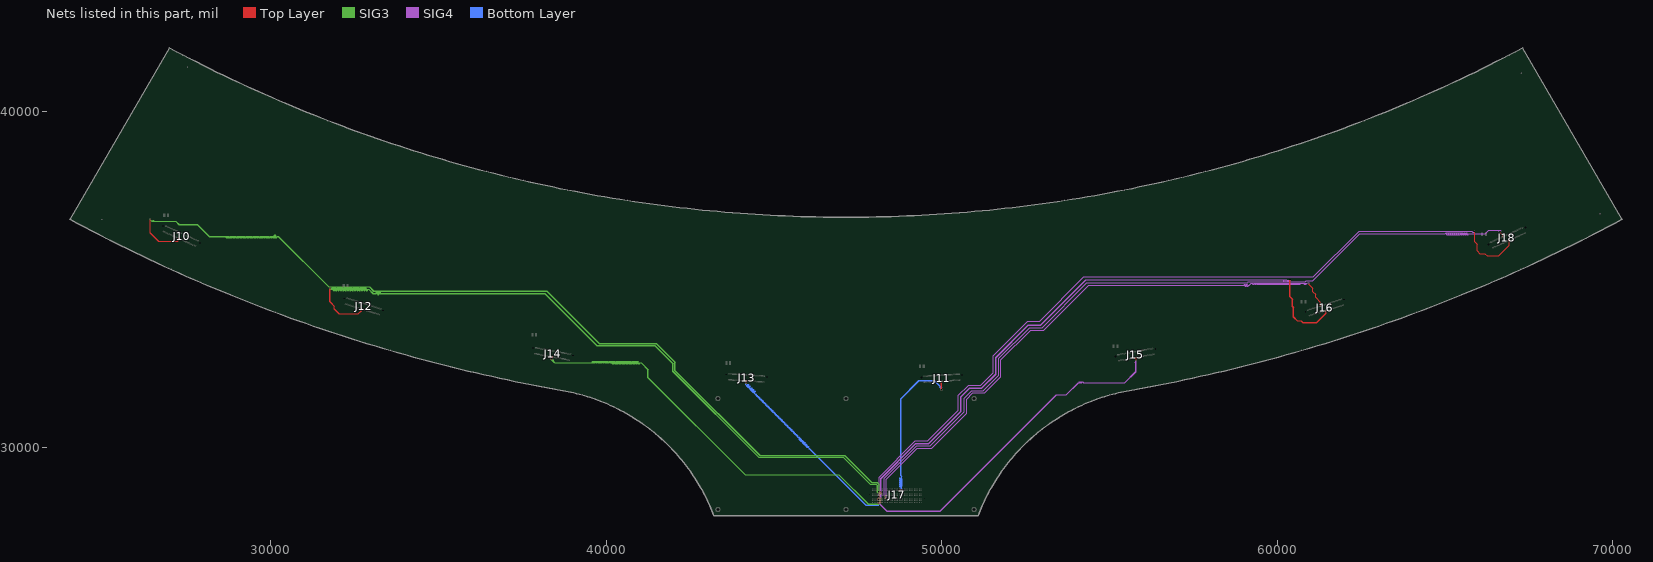
[diagram p0: the nets of this part, all layers, seen from the top]
# Altium PCB MISC86329.PcbDoc (part 9 of 11)
Units mil, origin at the board's own origin, x right, y up, seen from the top; angles counter-clockwise.
Board outline 46247.15 x 13937.21 mil, 6 copper layers (Top Layer, GND2, SIG3, SIG4, POWER5, Bottom Layer); 17 components, 210 nets, 908 pads, 1109 vias.

## Via types
v1: diameter 24, hole 12, Top Layer to Bottom Layer, 684 vias
v2: diameter 18, hole 9, Top Layer to Bottom Layer, 425 vias

## Nets (pads, with @x,y where several pads share a name; then routed paths per layer and width w, separated by ;. In a path a pad name is that pad's centre, name@x,y a point inside that pad or via, vN(x,y) a via of type N, cw(c..) or ccw(c..) an arc to the next point about the centre after c; other vN are vias at no path point) (continued)
DATAIN6P_CH6: J16.28 J17.D22 | length 18290.3
  Top Layer w5: v2(48314.09,28495) J17.D22@48337.89,28518.8 ; 60949,34880.5 60949,34846 61055,34740 61055,34648 61141,34562 61141,34474 61286,34329 61286,34220.6 J16.28@61285.27,34219.87
  SIG4 w5: v2(48314.09,28495) 48344,28524.91 48344,29053 49268,29977 49697.14,29977 50747,31026.86 50747,31446 50928,31627 51285.14,31627 51764,32105.86 51764,32612 52653,33501 53046.14,33501 54377.14,34832 59009.14,34832 59019.57,34842.43 59019.57,34857.43 59024.14,34862 59035,34862 59039.57,34857.43 59039.57,34812.43 59050,34802 59069.14,34802 59079.57,34812.43 59079.57,34857.43 59084.14,34862 59095,34862 59099.57,34857.43 59099.57,34812.43 59110,34802 59129.14,34802 59139.57,34812.43 59139.57,34827.43 59144.14,34832 59159.14,34832 59218.14,34891 59260.93,34891 59265.5,34886.43 59265.5,34871.43 59275.93,34861 59295.07,34861 59305.5,34871.43 59305.5,34886.43 59310.07,34891 59320.93,34891 59325.5,34886.43 59325.5,34871.43 59335.93,34861 59355.07,34861 59365.5,34871.43 59365.5,34886.43 59370.07,34891 59380.93,34891 59385.5,34886.43 59385.5,34871.43 59395.93,34861 59415.07,34861 59425.5,34871.43 59425.5,34886.43 59430.07,34891 59440.93,34891 59445.5,34886.43 59445.5,34871.43 59455.93,34861 59475.07,34861 59485.5,34871.43 59485.5,34886.43 59490.07,34891 59500.93,34891 59505.5,34886.43 59505.5,34871.43 59515.93,34861 59535.07,34861 59545.5,34871.43 59545.5,34886.43 59550.07,34891 59560.93,34891 59565.5,34886.43 59565.5,34871.43 59575.93,34861 59595.07,34861 59605.5,34871.43 59605.5,34886.43 59610.07,34891 59620.93,34891 59625.5,34886.43 59625.5,34871.43 59635.93,34861 59655.07,34861 59665.5,34871.43 59665.5,34886.43 59670.07,34891 59680.93,34891 59685.5,34886.43 59685.5,34871.43 59695.93,34861 59715.07,34861 59725.5,34871.43 59725.5,34886.43 59730.07,34891 59740.93,34891 59745.5,34886.43 59745.5,34871.43 59755.93,34861 59775.07,34861 59785.5,34871.43 59785.5,34886.43 59790.07,34891 59800.93,34891 59805.5,34886.43 59805.5,34871.43 59815.93,34861 59835.07,34861 59845.5,34871.43 59845.5,34886.43 59850.07,34891 59860.93,34891 59865.5,34886.43 59865.5,34871.43 59875.93,34861 59895.07,34861 59905.5,34871.43 59905.5,34886.43 59910.07,34891 59920.93,34891 59925.5,34886.43 59925.5,34871.43 59935.93,34861 59955.07,34861 59965.5,34871.43 59965.5,34886.43 59970.07,34891 59980.93,34891 59985.5,34886.43 59985.5,34871.43 59995.93,34861 60015.07,34861 60025.5,34871.43 60025.5,34886.43 60030.07,34891 60040.93,34891 60045.5,34886.43 60045.5,34871.43 60055.93,34861 60075.07,34861 60085.5,34871.43 60085.5,34886.43 60090.07,34891 60100.93,34891 60105.5,34886.43 60105.5,34871.43 60115.93,34861 60135.07,34861 60145.5,34871.43 60145.5,34886.43 60150.07,34891 60160.93,34891 60165.5,34886.43 60165.5,34871.43 60175.93,34861 60195.07,34861 60205.5,34871.43 60205.5,34886.43 60210.07,34891 60220.93,34891 60225.5,34886.43 60225.5,34871.43 60235.93,34861 60255.07,34861 60265.5,34871.43 60265.5,34886.43 60270.07,34891 60280.93,34891 60285.5,34886.43 60285.5,34871.43 60295.93,34861 60315.07,34861 60325.5,34871.43 60325.5,34886.43 60330.07,34891 60340.93,34891 60345.5,34886.43 60345.5,34871.43 60355.93,34861 60375.07,34861 60385.5,34871.43 60385.5,34886.43 60390.07,34891 60400.93,34891 60405.5,34886.43 60405.5,34871.43 60415.93,34861 60435.07,34861 60445.5,34871.43 60445.5,34886.43 60450.07,34891 60460.93,34891 60465.5,34886.43 60465.5,34871.43 60475.93,34861 60495.07,34861 60505.5,34871.43 60505.5,34886.43 60510.07,34891 60520.93,34891 60525.5,34886.43 60525.5,34871.43 60535.93,34861 60555.07,34861 60565.5,34871.43 60565.5,34886.43 60570.07,34891 60580.93,34891 60585.5,34886.43 60585.5,34871.43 60595.93,34861 60615.07,34861 60625.5,34871.43 60625.5,34886.43 60630.07,34891 60640.93,34891 60645.5,34886.43 60645.5,34871.43 60655.93,34861 60675.07,34861 60685.5,34871.43 60685.5,34886.43 60690.07,34891 60703,34891 60791,34891 60796,34886 60796,34873.23 60801,34868.23 60811,34868.23 60816,34873.23 60816,34886 60821,34891 60831,34891 60836,34886 60836,34873.23 60841,34868.23 60851,34868.23 60856,34873.23 60856,34886 60861,34891 60866,34891 60882.14,34891 60908.14,34917 60941,34917 60949,34909 60949,34893 v2@60943,34887
  other v2: 60942.5,34887
DATAIN6P_CH7: J17.E22 J18.28 | length 23893.1
  Top Layer w5: v2(48314.09,28545) J17.E22@48337.89,28568.8 ; 66665,36423.5 66665,36390 66717.39,36337.61 J18.28@66717.39,36281.33
  SIG4 w5: v2(48314.09,28545) 48294.09,28565 48294.09,29081.09 49260,30047 49655.14,30047 50669,31060.86 50669,31464.86 50895.14,31691 51236.14,31691 51698,32152.86 51698,32656 52618,33576 52990.14,33576 54328.14,34914 59117.14,34914 59137.14,34934 60830.14,34934 60868.14,34972 61057.14,34972 62452.14,36367 65008,36367 65038,36397 65049.43,36397 65054,36392.43 65054,36347.43 65064.43,36337 65083.57,36337 65094,36347.43 65094,36392.43 65098.57,36397 65109.43,36397 65114,36392.43 65114,36347.43 65124.43,36337 65143.57,36337 65154,36347.43 65154,36392.43 65158.57,36397 65169.43,36397 65174,36392.43 65174,36347.43 65184.43,36337 65203.57,36337 65214,36347.43 65214,36392.43 65218.57,36397 65229.43,36397 65234,36392.43 65234,36347.43 65244.43,36337 65263.57,36337 65274,36347.43 65274,36392.43 65278.57,36397 65289.43,36397 65294,36392.43 65294,36347.43 65304.43,36337 65323.57,36337 65334,36347.43 65334,36392.43 65338.57,36397 65349.43,36397 65354,36392.43 65354,36347.43 65364.43,36337 65383.57,36337 65394,36347.43 65394,36392.43 65398.57,36397 65409.43,36397 65414,36392.43 65414,36347.43 65424.43,36337 65443.57,36337 65454,36347.43 65454,36392.43 65458.57,36397 65469.43,36397 65474,36392.43 65474,36347.43 65484.43,36337 65503.57,36337 65514,36347.43 65514,36392.43 65518.57,36397 65529.43,36397 65534,36392.43 65534,36347.43 65544.43,36337 65563.57,36337 65574,36347.43 65574,36392.43 65578.57,36397 65589.43,36397 65594,36392.43 65594,36347.43 65604.43,36337 65623.57,36337 65634,36347.43 65634,36392.43 65638.57,36397 65649.43,36397 65654,36392.43 65654,36347.43 65664.43,36337 65683.57,36337 65694,36347.43 65694,36362.43 65698.57,36367 66189.14,36367 66304.14,36482 66581,36482 66586,36477 66586,36461.86 66591,36456.86 66601,36456.86 66606,36461.86 66606,36477 66611,36482 66637,36482 66665,36454 66665,36437 v2@66660,36432
  other v2: 66658.5,36430
DATAIN7N_CH0: J10.35 J17.G26 | length 28227.4
  Top Layer w5: v2(26406.5,36813) 26413,36806.5 26413,36389.86 26659.86,36143 27230.14,36143 27272.65,36185.51 27272.65,36199.68 J10.35@27291.29,36218.32 ; v2(48114.09,28692.61) J17.G26@48137.89,28668.8
  SIG3 w5: 26413,36806.5 26413,36783 26459,36737 27176,36737 27272,36641 27815.86,36641 27868.86,36588 ; 27869,36588 27868.86,36588 ; v2(48114.09,28692.61) 48134.09,28712.61 48134.09,28890.77 48073.86,28951 47916.86,28951 47107.86,29760 44584.86,29760 42053,32291.86 42053,32541 41497,33097 39794.86,33097 38227.86,34664 33067.86,34664 32946.86,34785 31734,34785 30233,36286 30200.32,36286 30194.5,36280.18 30194.5,36257.84 30182.82,36246.16 30161.18,36246.16 30149.5,36257.84 30149.5,36320.02 30143.68,36325.84 30130.32,36325.84 30124.5,36320.02 30124.5,36257.84 30112.82,36246.16 30091.18,36246.16 30079.5,36257.84 30079.5,36280.18 30073.68,36286 30060.32,36286 30054.5,36280.18 30054.5,36257.84 30042.82,36246.16 30021.18,36246.16 30009.5,36257.84 30009.5,36280.18 30003.68,36286 29990.32,36286 29984.5,36280.18 29984.5,36257.84 29972.82,36246.16 29951.18,36246.16 29939.5,36257.84 29939.5,36280.18 29933.68,36286 29920.32,36286 29914.5,36280.18 29914.5,36257.84 29902.82,36246.16 29881.18,36246.16 29869.5,36257.84 29869.5,36280.18 29863.68,36286 29850.32,36286 29844.5,36280.18 29844.5,36257.84 29832.82,36246.16 29811.18,36246.16 29799.5,36257.84 29799.5,36280.18 29793.68,36286 29780.32,36286 29774.5,36280.18 29774.5,36257.84 29762.82,36246.16 29741.18,36246.16 29729.5,36257.84 29729.5,36280.18 29723.68,36286 29710.32,36286 29704.5,36280.18 29704.5,36257.84 29692.82,36246.16 29671.18,36246.16 29659.5,36257.84 29659.5,36280.18 29653.68,36286 29640.32,36286 29634.5,36280.18 29634.5,36257.84 29622.82,36246.16 29601.18,36246.16 29589.5,36257.84 29589.5,36280.18 29583.68,36286 29570.32,36286 29564.5,36280.18 29564.5,36257.84 29552.82,36246.16 29531.18,36246.16 29519.5,36257.84 29519.5,36280.18 29513.68,36286 29500.32,36286 29494.5,36280.18 29494.5,36257.84 29482.82,36246.16 29461.18,36246.16 29449.5,36257.84 29449.5,36280.18 29443.68,36286 29430.32,36286 29424.5,36280.18 29424.5,36257.84 29412.82,36246.16 29391.18,36246.16 29379.5,36257.84 29379.5,36280.18 29373.68,36286 29360.32,36286 29354.5,36280.18 29354.5,36257.84 29342.82,36246.16 29321.18,36246.16 29309.5,36257.84 29309.5,36280.18 29303.68,36286 29290.32,36286 29284.5,36280.18 29284.5,36257.84 29272.82,36246.16 29251.18,36246.16 29239.5,36257.84 29239.5,36280.18 29233.68,36286 29220.32,36286 29214.5,36280.18 29214.5,36257.84 29202.82,36246.16 29181.18,36246.16 29169.5,36257.84 29169.5,36280.18 29163.68,36286 29150.32,36286 29144.5,36280.18 29144.5,36257.84 29132.82,36246.16 29111.18,36246.16 29099.5,36257.84 29099.5,36280.18 29093.68,36286 29080.32,36286 29074.5,36280.18 29074.5,36257.84 29062.82,36246.16 29041.18,36246.16 29029.5,36257.84 29029.5,36280.18 29023.68,36286 29010.32,36286 29004.5,36280.18 29004.5,36257.84 28992.82,36246.16 28971.18,36246.16 28959.5,36257.84 28959.5,36280.18 28953.68,36286 28940.32,36286 28934.5,36280.18 28934.5,36257.84 28922.82,36246.16 28901.18,36246.16 28889.5,36257.84 28889.5,36280.18 28883.68,36286 28870.32,36286 28864.5,36280.18 28864.5,36257.84 28852.82,36246.16 28831.18,36246.16 28819.5,36257.84 28819.5,36280.18 28813.68,36286 28800.32,36286 28794.5,36280.18 28794.5,36257.84 28782.82,36246.16 28761.18,36246.16 28749.5,36257.84 28749.5,36280.18 28743.68,36286 28730.32,36286 28724.5,36280.18 28724.5,36257.84 28712.82,36246.16 28691.18,36246.16 28679.5,36257.84 28679.5,36280.18 28673.68,36286 28170.86,36286 27868.86,36588
DATAIN7N_CH1: J12.35 J17.F26 | length 23092.2
  Top Layer w5: v2(31758.5,34755) 31765,34748.5 31765,34343.86 31895,34213.86 31895,34128.86 32039.86,33984 32619.14,33984 32713.22,34078.08 32713.22,34102.04 J12.35@32733.25,34122.07 ; v2(48114.09,28642.61) J17.F26@48137.89,28618.8
  SIG3 w5: v2(31758.5,34755) 31765,34748.5 31765,34729.86 31780.93,34713.93 ; 31781,34714 31783,34712 31830.82,34712 31842.5,34723.68 31842.5,34746.18 31848.32,34752 31861.68,34752 31867.5,34746.18 31867.5,34683.68 31879.18,34672 31900.82,34672 31912.5,34683.68 31912.5,34746.18 31918.32,34752 31931.68,34752 31937.5,34746.18 31937.5,34683.68 31949.18,34672 31970.82,34672 31982.5,34683.68 31982.5,34746.18 31988.32,34752 32001.68,34752 32007.5,34746.18 32007.5,34683.68 32019.18,34672 32040.82,34672 32052.5,34683.68 32052.5,34746.18 32058.32,34752 32071.68,34752 32077.5,34746.18 32077.5,34683.68 32089.18,34672 32110.82,34672 32122.5,34683.68 32122.5,34746.18 32128.32,34752 32141.68,34752 32147.5,34746.18 32147.5,34683.68 32159.18,34672 32180.82,34672 32192.5,34683.68 32192.5,34746.18 32198.32,34752 32211.68,34752 32217.5,34746.18 32217.5,34683.68 32229.18,34672 32250.82,34672 32262.5,34683.68 32262.5,34746.18 32268.32,34752 32281.68,34752 32287.5,34746.18 32287.5,34683.68 32299.18,34672 32320.82,34672 32332.5,34683.68 32332.5,34746.18 32338.32,34752 32351.68,34752 32357.5,34746.18 32357.5,34683.68 32369.18,34672 32390.82,34672 32402.5,34683.68 32402.5,34746.18 32408.32,34752 32421.68,34752 32427.5,34746.18 32427.5,34683.68 32439.18,34672 32460.82,34672 32472.5,34683.68 32472.5,34746.18 32478.32,34752 32491.68,34752 32497.5,34746.18 32497.5,34683.68 32509.18,34672 32530.82,34672 32542.5,34683.68 32542.5,34746.18 32548.32,34752 32561.68,34752 32567.5,34746.18 32567.5,34683.68 32579.18,34672 32600.82,34672 32612.5,34683.68 32612.5,34746.18 32618.32,34752 32631.68,34752 32637.5,34746.18 32637.5,34683.68 32649.18,34672 32670.82,34672 32682.5,34683.68 32682.5,34746.18 32688.32,34752 32701.68,34752 32707.5,34746.18 32707.5,34683.68 32719.18,34672 32740.82,34672 32752.5,34683.68 32752.5,34746.18 32758.32,34752 32771.68,34752 32777.5,34746.18 32777.5,34683.68 32789.18,34672 32810.82,34672 32822.5,34683.68 32822.5,34746.18 32828.32,34752 32841.68,34752 32847.5,34746.18 32847.5,34683.68 32859.18,34672 32880.82,34672 32892.5,34683.68 32892.5,34706.18 32898.32,34712 32930.86,34712 33052.86,34590 33155.82,34590 33167.5,34601.68 33167.5,34621.05 33173.32,34626.87 33186.68,34626.87 33192.5,34621.05 33192.5,34564.81 33204.18,34553.13 33225.82,34553.13 33237.5,34564.81 33237.5,34621.05 33243.32,34626.87 33256.68,34626.87 33262.5,34621.05 33262.5,34601.68 33274.18,34590 38166.86,34590 39724.86,33032 41451,33032 41987,32496 41987,32265.86 44547.86,29705 47065.86,29705 47870.86,28900 48045.86,28900 48086,28859.86 48086,28670.69 48104.66,28652.04 v2(48114.09,28642.61)
DATAIN7N_CH2: J14.35 J17.B26 | length 13805.7
  Top Layer w5: v2@38383.5,32646 38383.5,32645.67 v2(38383.83,32646) ; v2@38384,32646 38377,32653 38377,32676 38390.12,32689.12 J14.35@38390.12,32704.64 ; v2(48114.09,28395) J17.B26@48137.89,28418.8
  SIG3 w5: v2@38382,32643 38377,32638 38377,32625.14 38390.07,32612.07 38394.49,32607.65 38403.33,32607.65 38409.83,32614.15 38418.67,32614.15 38427.51,32605.31 38427.51,32596.47 38421.01,32589.97 38421.01,32581.14 38455.07,32547.07 38469.14,32533 39580.68,32533 39586.5,32538.82 39586.5,32561.32 39598.18,32573 39619.82,32573 39631.5,32561.32 39631.5,32538.82 39637.32,32533 39650.68,32533 39656.5,32538.82 39656.5,32561.32 39668.18,32573 39689.82,32573 39701.5,32561.32 39701.5,32538.82 39707.32,32533 39720.68,32533 39726.5,32538.82 39726.5,32561.32 39738.18,32573 39759.82,32573 39771.5,32561.32 39771.5,32538.82 39777.32,32533 39790.68,32533 39796.5,32538.82 39796.5,32561.32 39808.18,32573 39829.82,32573 39841.5,32561.32 39841.5,32538.82 39847.32,32533 39860.68,32533 39866.5,32538.82 39866.5,32561.32 39878.18,32573 39899.82,32573 39911.5,32561.32 39911.5,32538.82 39917.32,32533 39930.68,32533 39936.5,32538.82 39936.5,32561.32 39948.18,32573 39969.82,32573 39981.5,32561.32 39981.5,32538.82 39987.32,32533 40000.68,32533 40006.5,32538.82 40006.5,32561.32 40018.18,32573 40039.82,32573 40051.5,32561.32 40051.5,32538.82 40057.32,32533 40070.68,32533 40076.5,32538.82 40076.5,32561.32 40088.18,32573 40109.82,32573 40121.5,32561.32 40121.5,32538.82 40127.32,32533 40140.68,32533 40146.5,32538.82 40146.5,32561.32 40158.18,32573 40179.82,32573 40191.5,32561.32 40191.5,32508.82 40197.32,32503 40210.68,32503 40216.5,32508.82 40216.5,32561.32 40228.18,32573 40249.82,32573 40261.5,32561.32 40261.5,32508.82 40267.32,32503 40280.68,32503 40286.5,32508.82 40286.5,32561.32 40298.18,32573 40319.82,32573 40331.5,32561.32 40331.5,32508.82 40337.32,32503 40350.68,32503 40356.5,32508.82 40356.5,32561.32 40368.18,32573 40389.82,32573 40401.5,32561.32 40401.5,32508.82 40407.32,32503 40420.68,32503 40426.5,32508.82 40426.5,32561.32 40438.18,32573 40459.82,32573 40471.5,32561.32 40471.5,32508.82 40477.32,32503 40490.68,32503 40496.5,32508.82 40496.5,32561.32 40508.18,32573 40529.82,32573 40541.5,32561.32 40541.5,32508.82 40547.32,32503 40560.68,32503 40566.5,32508.82 40566.5,32561.32 40578.18,32573 40599.82,32573 40611.5,32561.32 40611.5,32508.82 40617.32,32503 40630.68,32503 40636.5,32508.82 40636.5,32561.32 40648.18,32573 40669.82,32573 40681.5,32561.32 40681.5,32508.82 40687.32,32503 40700.68,32503 40706.5,32508.82 40706.5,32561.32 40718.18,32573 40739.82,32573 40751.5,32561.32 40751.5,32508.82 40757.32,32503 40770.68,32503 40776.5,32508.82 40776.5,32561.32 40788.18,32573 40809.82,32573 40821.5,32561.32 40821.5,32508.82 40827.32,32503 40840.68,32503 40846.5,32508.82 40846.5,32561.32 40858.18,32573 40879.82,32573 40891.5,32561.32 40891.5,32508.82 40897.32,32503 40910.68,32503 40916.5,32508.82 40916.5,32561.32 40928.18,32573 40949.82,32573 40961.5,32561.32 40961.5,32508.82 40967.32,32503 40980.68,32503 40986.5,32508.82 40986.5,32521.32 40998.18,32533 41048,32533 41255,32326 41255,32084 44144,29195 46934,29195 47809,28320 48118,28320 48134,28336 48134,28375.09 v2(48114.09,28395)
DATAIN7N_CH3: J13.35 J17.A26 | length 7746.6
  Top Layer w5: 44166.84,31931.5 44166.84,31949.28 44177.55,31960 J13.35@44177.55,31987.19 ; v2(48114.09,28345) J17.A26@48137.89,28368.8
  Bottom Layer w5: v2@44172,31923 44167,31918 44167,31870.14 44183.03,31854.11 44188.79,31854.11 44221.32,31886.64 44235.36,31886.64 44253.14,31868.86 44253.14,31854.82 44220.61,31822.29 44220.61,31816.53 44232.53,31804.61 44238.29,31804.61 44270.81,31837.14 44284.85,31837.14 44302.63,31819.36 44302.63,31805.32 44270.11,31772.79 44270.11,31767.04 44282.03,31755.12 44287.78,31755.12 44320.31,31787.64 44334.35,31787.64 44352.13,31769.86 44352.13,31755.82 44319.6,31723.3 44319.6,31717.54 44331.52,31705.62 44337.28,31705.62 44369.81,31738.15 44383.85,31738.15 44401.63,31720.37 44401.63,31706.33 44369.1,31673.8 44369.1,31668.04 44381.02,31656.12 44386.78,31656.12 44419.31,31688.65 44433.35,31688.65 44451.13,31670.87 44451.13,31656.83 44418.6,31624.3 44418.6,31618.54 44443.41,31593.73 44446.34,31593.73 44453.41,31600.8 44464.62,31600.8 44478.16,31587.27 44478.16,31576.05 44471.09,31568.98 44471.09,31566.05 44478.77,31558.38 44481.69,31558.38 44488.77,31565.45 44499.98,31565.45 44513.51,31551.91 44513.51,31540.7 44506.44,31533.63 44506.44,31530.7 44514.12,31523.02 44517.05,31523.02 44524.12,31530.09 44535.33,31530.09 44548.87,31516.56 44548.87,31505.34 44541.8,31498.27 44541.8,31495.34 44549.48,31487.67 44552.4,31487.67 44559.48,31494.74 44570.69,31494.74 44584.22,31481.2 44584.22,31469.99 44577.15,31462.92 44577.15,31459.99 44584.83,31452.31 44587.76,31452.31 44594.83,31459.38 44606.04,31459.38 44619.58,31445.85 44619.58,31434.63 44612.51,31427.56 44612.51,31424.63 44620.19,31416.96 44623.12,31416.96 44630.19,31424.03 44641.4,31424.03 44654.94,31410.49 44654.94,31399.28 44647.86,31392.21 44647.86,31389.28 44655.54,31381.6 44658.47,31381.6 44665.54,31388.67 44676.76,31388.67 44690.29,31375.14 44690.29,31363.92 44683.22,31356.85 44683.22,31353.92 44690.9,31346.24 44693.83,31346.24 44700.9,31353.32 44712.11,31353.32 44725.65,31339.78 44725.65,31328.57 44718.57,31321.5 44718.57,31318.57 44726.25,31310.89 44729.18,31310.89 44736.25,31317.96 44747.47,31317.96 44761,31304.43 44761,31293.21 44753.93,31286.14 44753.93,31283.21 44761.61,31275.53 44764.54,31275.53 44771.61,31282.61 44782.82,31282.61 44796.36,31269.07 44796.36,31257.86 44789.29,31250.79 44789.29,31247.86 44796.96,31240.18 44799.89,31240.18 44806.96,31247.25 44818.18,31247.25 44831.71,31233.71 44831.71,31222.5 44824.64,31215.43 44824.64,31212.5 44832.32,31204.82 44835.25,31204.82 44842.32,31211.89 44853.53,31211.89 44867.07,31198.36 44867.07,31187.15 44860,31180.07 44860,31177.15 44867.67,31169.47 44870.6,31169.47 44877.67,31176.54 44888.89,31176.54 44902.42,31163 44902.42,31151.79 44895.35,31144.72 44895.35,31141.79 44903.03,31134.11 44905.96,31134.11 44913.03,31141.18 44924.24,31141.18 44937.78,31127.65 44937.78,31116.44 44930.71,31109.36 44930.71,31106.44 44938.38,31098.76 44941.31,31098.76 44948.38,31105.83 44959.6,31105.83 44973.13,31092.29 44973.13,31081.08 44966.06,31074.01 44966.06,31071.08 44973.74,31063.4 44976.67,31063.4 44983.74,31070.47 44994.95,31070.47 45008.49,31056.94 45008.49,31045.72 45001.42,31038.65 45001.42,31035.72 45009.1,31028.05 45012.02,31028.05 45019.1,31035.12 45030.31,31035.12 45043.84,31021.58 45043.84,31010.37 45036.77,31003.3 45036.77,31000.37 45044.45,30992.69 45047.38,30992.69 45054.45,30999.76 45065.66,30999.76 45079.2,30986.23 45079.2,30975.01 45072.13,30967.94 45072.13,30965.01 45079.81,30957.34 45082.73,30957.34 45089.81,30964.41 45101.02,30964.41 45114.55,30950.87 45114.55,30939.66 45107.48,30932.59 45107.48,30929.66 45115.16,30921.98 45118.09,30921.98 45125.16,30929.05 45136.37,30929.05 45149.91,30915.52 45149.91,30904.3 45142.84,30897.23 45142.84,30894.3 45150.52,30886.63 45153.45,30886.63 45160.52,30893.7 45171.73,30893.7 45185.27,30880.16 45185.27,30868.95 45178.19,30861.88 45178.19,30858.95 45185.87,30851.27 45188.8,30851.27 45195.87,30858.34 45207.09,30858.34 45220.62,30844.81 45220.62,30833.59 45213.55,30826.52 45213.55,30823.59 45221.23,30815.91 45224.16,30815.91 45231.23,30822.99 45242.44,30822.99 45255.98,30809.45 45255.98,30798.24 45248.9,30791.17 45248.9,30788.24 45256.58,30780.56 45259.51,30780.56 45266.58,30787.63 45277.8,30787.63 45291.33,30774.1 45291.33,30762.88 45284.26,30755.81 45284.26,30752.88 45291.94,30745.2 45294.87,30745.2 45301.94,30752.28 45313.15,30752.28 45326.69,30738.74 45326.69,30727.53 45319.62,30720.46 45319.62,30717.53 45327.29,30709.85 45330.22,30709.85 45337.29,30716.92 45348.51,30716.92 45362.04,30703.38 45362.04,30692.17 45354.97,30685.1 45354.97,30682.17 45362.65,30674.49 45365.58,30674.49 45372.65,30681.56 45383.86,30681.56 45397.4,30668.03 45397.4,30656.82 45390.33,30649.74 45390.33,30646.82 45398,30639.14 45400.93,30639.14 45408,30646.21 45419.22,30646.21 45432.75,30632.67 45432.75,30621.46 45425.68,30614.39 45425.68,30611.46 45433.36,30603.78 45436.29,30603.78 45443.36,30610.85 45454.57,30610.85 45468.11,30597.32 45468.11,30586.1 45461.04,30579.03 45461.04,30576.1 45468.71,30568.43 45471.64,30568.43 45478.71,30575.5 45489.93,30575.5 45503.46,30561.96 45503.46,30550.75 45496.39,30543.68 45496.39,30540.75 45504.07,30533.07 45507,30533.07 45514.07,30540.14 45525.28,30540.14 45538.82,30526.61 45538.82,30515.39 45531.75,30508.32 45531.75,30505.39 45539.43,30497.72 45542.35,30497.72 45549.43,30504.79 45560.64,30504.79 45574.17,30491.25 45574.17,30480.04 45567.1,30472.97 45567.1,30470.04 45574.78,30462.36 45577.71,30462.36 45584.78,30469.43 45595.99,30469.43 45609.53,30455.9 45609.53,30444.68 45602.46,30437.61 45602.46,30434.68 45610.14,30427.01 45613.06,30427.01 45620.14,30434.08 45631.35,30434.08 45644.88,30420.54 45644.88,30409.33 45637.81,30402.26 45637.81,30399.33 45645.49,30391.65 45648.42,30391.65 45655.49,30398.72 45666.7,30398.72 45680.24,30385.19 45680.24,30373.97 45673.17,30366.9 45673.17,30363.97 45680.85,30356.3 45683.78,30356.3 45690.85,30363.37 45702.06,30363.37 45715.6,30349.83 45715.6,30338.62 45708.52,30331.55 45708.52,30328.62 45716.2,30320.94 45719.13,30320.94 45726.2,30328.01 45737.42,30328.01 45750.95,30314.48 45750.95,30303.26 45743.88,30296.19 45743.88,30293.26 45751.56,30285.58 45754.49,30285.58 45761.56,30292.66 45772.77,30292.66 45786.31,30279.12 45786.31,30267.91 45765.09,30246.69 45765.09,30243.76 45772.77,30236.09 45775.7,30236.09 45796.91,30257.3 45808.13,30257.3 45821.66,30243.76 45821.66,30232.55 45800.45,30211.34 45800.45,30208.41 45808.13,30200.73 45811.05,30200.73 45832.27,30221.94 45843.48,30221.94 45857.02,30208.41 45857.02,30197.2 45835.8,30175.98 45835.8,30173.05 45843.48,30165.38 45846.41,30165.38 45867.62,30186.59 45878.84,30186.59 45892.37,30173.05 45892.37,30161.84 45871.16,30140.63 45871.16,30137.7 45878.84,30130.02 45881.77,30130.02 45902.98,30151.23 45914.19,30151.23 45927.73,30137.7 45927.73,30126.49 45906.51,30105.27 45906.51,30102.34 45914.19,30094.67 45917.12,30094.67 45938.33,30115.88 45949.55,30115.88 45963.08,30102.34 45963.08,30091.13 45941.87,30069.92 45941.87,30066.99 45949.55,30059.31 45952.48,30059.31 45973.69,30080.52 45984.9,30080.52 45998.44,30066.99 45998.44,30055.77 45977.22,30034.56 45977.22,30031.63 45984.9,30023.96 45987.83,30023.96 46009.04,30045.17 46020.26,30045.17 46034,30031.43 46034,29993.14 46049.14,29978 46059.14,29978 47742.14,28295 48018,28295 48024,28295 48028,28299 48028,28311 48032,28315 48044,28315 48048,28311 48048,28299 48052,28295 48091,28295 48116.2,28295 48135,28313.8 48135,28324.09 v2(48114.09,28345)
  other v2: 44173.34,31925
DATAIN7N_CH4: J11.35 J17.H14 | length 5092.9
  Top Layer w5: J17.H14@48737.89,28718.8 v2(48761.69,28742.61) ; 49998.57,31728.5 49998.57,31944.28 50009.29,31955 J11.35@50009.29,31980.39
  Bottom Layer w5: v2(48761.69,28742.61) 48781.69,28762.61 48781.69,28823.43 48777.12,28828 48762.12,28828 48751.69,28838.43 48751.69,28857.57 48762.12,28868 48807.12,28868 48811.69,28872.57 48811.69,28883.43 48807.12,28888 48762.12,28888 48751.69,28898.43 48751.69,28917.57 48762.12,28928 48807.12,28928 48811.69,28932.57 48811.69,28943.43 48807.12,28948 48762.12,28948 48751.69,28958.43 48751.69,28977.57 48762.12,28988 48807.12,28988 48811.69,28992.57 48811.69,29003.43 48807.12,29008 48762.12,29008 48751.69,29018.43 48751.69,29037.57 48762.12,29048 48807.12,29048 48811.69,29052.57 48811.69,29063.43 48807.12,29068 48762.12,29068 48751.69,29078.43 48751.69,29097.57 48762.12,29108 48799.86,29108 48806,29114.14 48806,29129 48781.69,29153.31 48781.69,31456.69 49324,31999 49783.14,31999 49998,31784.14 49998,31729.41 49998.57,31728.83 49998.57,31728.43 v2@50005,31722
  other v2: 50005.07,31722
DATAIN7N_CH5: J15.35 J17.C26 | length 10125.3
  Top Layer w5: v2(48114.09,28445) J17.C26@48137.89,28468.8 ; 55794,32611.5 55794,32653.61 55798.39,32658 J15.35@55798.39,32684.35
  SIG4 w5: v2(48114.09,28445) 48134.09,28425 48134.09,28329.91 48358,28106 49963.14,28106 53425.14,31568 53719.14,31568 54077.14,31926 54105.57,31926 54116,31936.43 54116,31951.43 54120.57,31956 54131.43,31956 54136,31951.43 54136,31936.43 54146.43,31926 54165.57,31926 54176,31936.43 54176,31951.43 54180.57,31956 54192,31956 54222,31926 55456.14,31926 55795,32264.86 55795,32599 v2@55800,32604
  other v2: 55800.5,32605
DATAIN7N_CH6: J16.35 J17.D26 | length 18293.1
  Top Layer w5: v2(48114.09,28495) J17.D26@48137.89,28518.8 ; 60372,35005.5 60372,34495 60448,34419 60448,34200 60476,34172 60476,33887.86 60588.86,33775 60702.86,33775 60751.86,33726 61181.14,33726 61457,34001.86 61457,34060.46 ; 61458.54,34062 J16.35@61458.54,34088.58
  SIG4 w5: v2(48114.09,28495) 48140.75,28495 48157.25,28511.5 48166.44,28511.5 48182,28527.06 48182,29082.14 49226.86,30127 49613,30127 50570,31084 50570,31514.14 50835.86,31780 51194,31780 51609,32195 51609,32685.14 52581.86,33658 52949,33658 54297,35006 60269.14,35006 60293.14,34982 60361,34982 60371,34992 60371,35004 v2@60366,35009
  other v2: 60365.5,35012
DATAIN7N_CH7: J17.E26 J18.35 | length 23899
  Top Layer w5: v2(48114.09,28545) J17.E26@48137.89,28568.8 ; v2(65879.5,36445) 65886,36438.5 65886,36129 65960,36055 65960,35859.86 66038.86,35781 66179.86,35781 66250.86,35710 66593.14,35710 66908,36024.86 66908,36141.95 66905.16,36144.79 66905.37,36145 J18.35@66905.37,36172.14
  SIG4 w5: v2(48114.09,28545) 48134.09,28565 48134.09,29119.23 49210.86,30196 49583,30196 50497,31110 50497,31552.14 50802.86,31858 51164,31858 51542,32236 51542,32739.14 52566.86,33764 52918,33764 54240,35086 61073,35086 62437,36450 65791,36450 65820,36421 65877.86,36421 65885,36428.14 65885,36439.5 v2(65879.5,36445)
DATAIN7P_CH0: J10.33 J17.G25 | length 28226.6
  Top Layer w5: v2(26429.5,36813) 26423,36806.5 26423,36394 26664,36153 27226,36153 27262.65,36189.65 J10.33@27262.65,36231.42 ; v2(48164.09,28692.61) J17.G25@48187.89,28668.8
  SIG3 w5: 26423,36806.5 26423,36787.14 26463.14,36747 26487,36747 26492,36747 26497,36752 26497,36761.4 26502,36766.4 26512,36766.4 26517,36761.4 26517,36752 26522,36747 26662,36747 27180.14,36747 27276.14,36651 27820.14,36651 27879,36592.14 27879,36592 28175,36296 28677.82,36296 28689.5,36284.32 28689.5,36261.98 28695.32,36256.16 28708.68,36256.16 28714.5,36261.98 28714.5,36284.32 28726.18,36296 28747.82,36296 28759.5,36284.32 28759.5,36261.98 28765.32,36256.16 28778.68,36256.16 28784.5,36261.98 28784.5,36284.32 28796.18,36296 28817.82,36296 28829.5,36284.32 28829.5,36261.98 28835.32,36256.16 28848.68,36256.16 28854.5,36261.98 28854.5,36284.32 28866.18,36296 28887.82,36296 28899.5,36284.32 28899.5,36261.98 28905.32,36256.16 28918.68,36256.16 28924.5,36261.98 28924.5,36284.32 28936.18,36296 28957.82,36296 28969.5,36284.32 28969.5,36261.98 28975.32,36256.16 28988.68,36256.16 28994.5,36261.98 28994.5,36284.32 29006.18,36296 29027.82,36296 29039.5,36284.32 29039.5,36261.98 29045.32,36256.16 29058.68,36256.16 29064.5,36261.98 29064.5,36284.32 29076.18,36296 29097.82,36296 29109.5,36284.32 29109.5,36261.98 29115.32,36256.16 29128.68,36256.16 29134.5,36261.98 29134.5,36284.32 29146.18,36296 29167.82,36296 29179.5,36284.32 29179.5,36261.98 29185.32,36256.16 29198.68,36256.16 29204.5,36261.98 29204.5,36284.32 29216.18,36296 29237.82,36296 29249.5,36284.32 29249.5,36261.98 29255.32,36256.16 29268.68,36256.16 29274.5,36261.98 29274.5,36284.32 29286.18,36296 29307.82,36296 29319.5,36284.32 29319.5,36261.98 29325.32,36256.16 29338.68,36256.16 29344.5,36261.98 29344.5,36284.32 29356.18,36296 29377.82,36296 29389.5,36284.32 29389.5,36261.98 29395.32,36256.16 29408.68,36256.16 29414.5,36261.98 29414.5,36284.32 29426.18,36296 29447.82,36296 29459.5,36284.32 29459.5,36261.98 29465.32,36256.16 29478.68,36256.16 29484.5,36261.98 29484.5,36284.32 29496.18,36296 29517.82,36296 29529.5,36284.32 29529.5,36261.98 29535.32,36256.16 29548.68,36256.16 29554.5,36261.98 29554.5,36284.32 29566.18,36296 29587.82,36296 29599.5,36284.32 29599.5,36261.98 29605.32,36256.16 29618.68,36256.16 29624.5,36261.98 29624.5,36284.32 29636.18,36296 29657.82,36296 29669.5,36284.32 29669.5,36261.98 29675.32,36256.16 29688.68,36256.16 29694.5,36261.98 29694.5,36284.32 29706.18,36296 29727.82,36296 29739.5,36284.32 29739.5,36261.98 29745.32,36256.16 29758.68,36256.16 29764.5,36261.98 29764.5,36284.32 29776.18,36296 29797.82,36296 29809.5,36284.32 29809.5,36261.98 29815.32,36256.16 29828.68,36256.16 29834.5,36261.98 29834.5,36284.32 29846.18,36296 29867.82,36296 29879.5,36284.32 29879.5,36261.98 29885.32,36256.16 29898.68,36256.16 29904.5,36261.98 29904.5,36284.32 29916.18,36296 29937.82,36296 29949.5,36284.32 29949.5,36261.98 29955.32,36256.16 29968.68,36256.16 29974.5,36261.98 29974.5,36284.32 29986.18,36296 30007.82,36296 30019.5,36284.32 30019.5,36261.98 30025.32,36256.16 30038.68,36256.16 30044.5,36261.98 30044.5,36284.32 30056.18,36296 30077.82,36296 30089.5,36284.32 30089.5,36261.98 30095.32,36256.16 30108.68,36256.16 30114.5,36261.98 30114.5,36324.16 30126.18,36335.84 30147.82,36335.84 30159.5,36324.16 30159.5,36261.98 30165.32,36256.16 30178.68,36256.16 30184.5,36261.98 30184.5,36284.32 30196.18,36296 30237.14,36296 31738.14,34795 32951,34795 33072,34674 38232,34674 39799,33107 41501.14,33107 42063,32545.14 42063,32296 44589,29770 47112,29770 47921,28961 48078,28961 48144.09,28894.91 48144.09,28712.61 v2(48164.09,28692.61)
DATAIN7P_CH1: J12.33 J17.F25 | length 23097.8
  Top Layer w5: v2(31781.5,34755) 31775,34748.5 31775,34348 31905,34218 31905,34133 32044,33994 32615,33994 32703.22,34082.22 J12.33@32703.22,34131.57 ; v2(48164.09,28642.61) J17.F25@48187.89,28618.8
  SIG3 w5: v2(31781.5,34755) 31775,34748.5 31775,34734 31775.14,34734 31787.14,34722 31826.68,34722 31832.5,34727.82 31832.5,34750.32 31844.18,34762 31865.82,34762 31877.5,34750.32 31877.5,34687.82 31883.32,34682 31896.68,34682 31902.5,34687.82 31902.5,34750.32 31914.18,34762 31935.82,34762 31947.5,34750.32 31947.5,34687.82 31953.32,34682 31966.68,34682 31972.5,34687.82 31972.5,34750.32 31984.18,34762 32005.82,34762 32017.5,34750.32 32017.5,34687.82 32023.32,34682 32036.68,34682 32042.5,34687.82 32042.5,34750.32 32054.18,34762 32075.82,34762 32087.5,34750.32 32087.5,34687.82 32093.32,34682 32106.68,34682 32112.5,34687.82 32112.5,34750.32 32124.18,34762 32145.82,34762 32157.5,34750.32 32157.5,34687.82 32163.32,34682 32176.68,34682 32182.5,34687.82 32182.5,34750.32 32194.18,34762 32215.82,34762 32227.5,34750.32 32227.5,34687.82 32233.32,34682 32246.68,34682 32252.5,34687.82 32252.5,34750.32 32264.18,34762 32285.82,34762 32297.5,34750.32 32297.5,34687.82 32303.32,34682 32316.68,34682 32322.5,34687.82 32322.5,34750.32 32334.18,34762 32355.82,34762 32367.5,34750.32 32367.5,34687.82 32373.32,34682 32386.68,34682 32392.5,34687.82 32392.5,34750.32 32404.18,34762 32425.82,34762 32437.5,34750.32 32437.5,34687.82 32443.32,34682 32456.68,34682 32462.5,34687.82 32462.5,34750.32 32474.18,34762 32495.82,34762 32507.5,34750.32 32507.5,34687.82 32513.32,34682 32526.68,34682 32532.5,34687.82 32532.5,34750.32 32544.18,34762 32565.82,34762 32577.5,34750.32 32577.5,34687.82 32583.32,34682 32596.68,34682 32602.5,34687.82 32602.5,34750.32 32614.18,34762 32635.82,34762 32647.5,34750.32 32647.5,34687.82 32653.32,34682 32666.68,34682 32672.5,34687.82 32672.5,34750.32 32684.18,34762 32705.82,34762 32717.5,34750.32 32717.5,34687.82 32723.32,34682 32736.68,34682 32742.5,34687.82 32742.5,34750.32 32754.18,34762 32775.82,34762 32787.5,34750.32 32787.5,34687.82 32793.32,34682 32806.68,34682 32812.5,34687.82 32812.5,34750.32 32824.18,34762 32845.82,34762 32857.5,34750.32 32857.5,34687.82 32863.32,34682 32876.68,34682 32882.5,34687.82 32882.5,34710.32 32894.18,34722 32935,34722 33057,34600 33151.68,34600 33157.5,34605.82 33157.5,34625.19 33169.18,34636.87 33190.82,34636.87 33202.5,34625.19 33202.5,34568.95 33208.32,34563.13 33221.68,34563.13 33227.5,34568.95 33227.5,34625.19 33239.18,34636.87 33260.82,34636.87 33272.5,34625.19 33272.5,34605.82 33278.32,34600 38171,34600 39729,33042 41455.14,33042 41997,32500.14 41997,32270 44552,29715 47070,29715 47875,28910 48050,28910 48096,28864 48096,28674.83 48111.73,28659.11 48120.92,28659.11 48137.42,28642.61 v2(48164.09,28642.61)
DATAIN7P_CH2: J14.33 J17.B25 | length 13806
  Top Layer w5: J14.33@38359.15,32710.42 38359.15,32684 38367,32676.15 38367,32652.5 ; v2(48164.09,28395) J17.B25@48187.89,28418.8
  SIG3 w5: v2@38361,32645 38367,32639 38367,32621 38383,32605 38387.42,32600.58 38413.94,32574.06 38448,32540 38465,32523 39584.82,32523 39596.5,32534.68 39596.5,32557.18 39602.32,32563 39615.68,32563 39621.5,32557.18 39621.5,32534.68 39633.18,32523 39654.82,32523 39666.5,32534.68 39666.5,32557.18 39672.32,32563 39685.68,32563 39691.5,32557.18 39691.5,32534.68 39703.18,32523 39724.82,32523 39736.5,32534.68 39736.5,32557.18 39742.32,32563 39755.68,32563 39761.5,32557.18 39761.5,32534.68 39773.18,32523 39794.82,32523 39806.5,32534.68 39806.5,32557.18 39812.32,32563 39825.68,32563 39831.5,32557.18 39831.5,32534.68 39843.18,32523 39864.82,32523 39876.5,32534.68 39876.5,32557.18 39882.32,32563 39895.68,32563 39901.5,32557.18 39901.5,32534.68 39913.18,32523 39934.82,32523 39946.5,32534.68 39946.5,32557.18 39952.32,32563 39965.68,32563 39971.5,32557.18 39971.5,32534.68 39983.18,32523 40004.82,32523 40016.5,32534.68 40016.5,32557.18 40022.32,32563 40035.68,32563 40041.5,32557.18 40041.5,32534.68 40053.18,32523 40074.82,32523 40086.5,32534.68 40086.5,32557.18 40092.32,32563 40105.68,32563 40111.5,32557.18 40111.5,32534.68 40123.18,32523 40144.82,32523 40156.5,32534.68 40156.5,32557.18 40162.32,32563 40175.68,32563 40181.5,32557.18 40181.5,32504.68 40193.18,32493 40214.82,32493 40226.5,32504.68 40226.5,32557.18 40232.32,32563 40245.68,32563 40251.5,32557.18 40251.5,32504.68 40263.18,32493 40284.82,32493 40296.5,32504.68 40296.5,32557.18 40302.32,32563 40315.68,32563 40321.5,32557.18 40321.5,32504.68 40333.18,32493 40354.82,32493 40366.5,32504.68 40366.5,32557.18 40372.32,32563 40385.68,32563 40391.5,32557.18 40391.5,32504.68 40403.18,32493 40424.82,32493 40436.5,32504.68 40436.5,32557.18 40442.32,32563 40455.68,32563 40461.5,32557.18 40461.5,32504.68 40473.18,32493 40494.82,32493 40506.5,32504.68 40506.5,32557.18 40512.32,32563 40525.68,32563 40531.5,32557.18 40531.5,32504.68 40543.18,32493 40564.82,32493 40576.5,32504.68 40576.5,32557.18 40582.32,32563 40595.68,32563 40601.5,32557.18 40601.5,32504.68 40613.18,32493 40634.82,32493 40646.5,32504.68 40646.5,32557.18 40652.32,32563 40665.68,32563 40671.5,32557.18 40671.5,32504.68 40683.18,32493 40704.82,32493 40716.5,32504.68 40716.5,32557.18 40722.32,32563 40735.68,32563 40741.5,32557.18 40741.5,32504.68 40753.18,32493 40774.82,32493 40786.5,32504.68 40786.5,32557.18 40792.32,32563 40805.68,32563 40811.5,32557.18 40811.5,32504.68 40823.18,32493 40844.82,32493 40856.5,32504.68 40856.5,32557.18 40862.32,32563 40875.68,32563 40881.5,32557.18 40881.5,32504.68 40893.18,32493 40914.82,32493 40926.5,32504.68 40926.5,32557.18 40932.32,32563 40945.68,32563 40951.5,32557.18 40951.5,32504.68 40963.18,32493 40984.82,32493 40996.5,32504.68 40996.5,32517.18 41002.32,32523 41043.86,32523 41245,32321.86 41245,32079.86 44139.86,29185 46929.86,29185 47804.86,28310 48122.14,28310 48144,28331.86 48144,28374.91 v2(48164.09,28395)
  other v2: 38360.5,32646
DATAIN7P_CH3: J13.33 J17.A25 | length 7748.9
  Top Layer w5: J13.33@44146.12,31989.15 44146.12,31960 44156.84,31949.28 44156.84,31931.5 ; v2(48164.09,28345) J17.A25@48187.89,28368.8
  Bottom Layer w5: v2@44153,31922 44157,31918 44157,31866 44178.89,31844.11 44192.93,31844.11 44225.46,31876.64 44231.21,31876.64 44243.14,31864.72 44243.14,31858.96 44210.61,31826.43 44210.61,31812.39 44228.39,31794.61 44242.43,31794.61 44274.96,31827.14 44280.71,31827.14 44292.63,31815.22 44292.63,31809.46 44260.11,31776.94 44260.11,31762.89 44277.88,31745.12 44291.93,31745.12 44324.45,31777.64 44330.21,31777.64 44342.13,31765.72 44342.13,31759.97 44309.6,31727.44 44309.6,31713.4 44327.38,31695.62 44341.42,31695.62 44373.95,31728.15 44379.71,31728.15 44391.63,31716.22 44391.63,31710.47 44359.1,31677.94 44359.1,31663.9 44376.88,31646.12 44390.92,31646.12 44423.45,31678.65 44429.2,31678.65 44441.13,31666.73 44441.13,31660.97 44408.6,31628.44 44408.6,31614.4 44439.27,31583.73 44450.48,31583.73 44457.55,31590.8 44460.48,31590.8 44468.16,31583.13 44468.16,31580.2 44461.09,31573.13 44461.09,31561.91 44474.62,31548.38 44485.84,31548.38 44492.91,31555.45 44495.84,31555.45 44503.51,31547.77 44503.51,31544.84 44496.44,31537.77 44496.44,31526.56 44509.98,31513.02 44521.19,31513.02 44528.26,31520.09 44531.19,31520.09 44538.87,31512.41 44538.87,31509.49 44531.8,31502.41 44531.8,31491.2 44545.33,31477.67 44556.55,31477.67 44563.62,31484.74 44566.55,31484.74 44574.22,31477.06 44574.22,31474.13 44567.15,31467.06 44567.15,31455.85 44580.69,31442.31 44591.9,31442.31 44598.97,31449.38 44601.9,31449.38 44609.58,31441.7 44609.58,31438.78 44602.51,31431.7 44602.51,31420.49 44616.04,31406.96 44627.26,31406.96 44634.33,31414.03 44637.26,31414.03 44644.94,31406.35 44644.94,31403.42 44637.86,31396.35 44637.86,31385.14 44651.4,31371.6 44662.61,31371.6 44669.68,31378.67 44672.61,31378.67 44680.29,31370.99 44680.29,31368.06 44673.22,31360.99 44673.22,31349.78 44686.75,31336.24 44697.97,31336.24 44705.04,31343.32 44707.97,31343.32 44715.65,31335.64 44715.65,31332.71 44708.57,31325.64 44708.57,31314.42 44722.11,31300.89 44733.32,31300.89 44740.39,31307.96 44743.32,31307.96 44751,31300.28 44751,31297.35 44743.93,31290.28 44743.93,31279.07 44757.47,31265.53 44768.68,31265.53 44775.75,31272.61 44778.68,31272.61 44786.36,31264.93 44786.36,31262 44779.29,31254.93 44779.29,31243.71 44792.82,31230.18 44804.03,31230.18 44811.11,31237.25 44814.03,31237.25 44821.71,31229.57 44821.71,31226.64 44814.64,31219.57 44814.64,31208.36 44828.18,31194.82 44839.39,31194.82 44846.46,31201.89 44849.39,31201.89 44857.07,31194.22 44857.07,31191.29 44850,31184.22 44850,31173 44863.53,31159.47 44874.74,31159.47 44881.82,31166.54 44884.75,31166.54 44892.42,31158.86 44892.42,31155.93 44885.35,31148.86 44885.35,31137.65 44898.89,31124.11 44910.1,31124.11 44917.17,31131.18 44920.1,31131.18 44927.78,31123.51 44927.78,31120.58 44920.71,31113.51 44920.71,31102.29 44934.24,31088.76 44945.46,31088.76 44952.53,31095.83 44955.46,31095.83 44963.13,31088.15 44963.13,31085.22 44956.06,31078.15 44956.06,31066.94 44969.6,31053.4 44980.81,31053.4 44987.88,31060.47 44990.81,31060.47 44998.49,31052.8 44998.49,31049.87 44991.42,31042.8 44991.42,31031.58 45004.95,31018.05 45016.17,31018.05 45023.24,31025.12 45026.17,31025.12 45033.84,31017.44 45033.84,31014.51 45026.77,31007.44 45026.77,30996.23 45040.31,30982.69 45051.52,30982.69 45058.59,30989.76 45061.52,30989.76 45069.2,30982.08 45069.2,30979.16 45062.13,30972.08 45062.13,30960.87 45075.66,30947.34 45086.88,30947.34 45093.95,30954.41 45096.88,30954.41 45104.55,30946.73 45104.55,30943.8 45097.48,30936.73 45097.48,30925.52 45111.02,30911.98 45122.23,30911.98 45129.3,30919.05 45132.23,30919.05 45139.91,30911.37 45139.91,30908.45 45132.84,30901.37 45132.84,30890.16 45146.37,30876.63 45157.59,30876.63 45164.66,30883.7 45167.59,30883.7 45175.27,30876.02 45175.27,30873.09 45168.19,30866.02 45168.19,30854.81 45181.73,30841.27 45192.94,30841.27 45200.01,30848.34 45202.94,30848.34 45210.62,30840.66 45210.62,30837.73 45203.55,30830.66 45203.55,30819.45 45217.09,30805.91 45228.3,30805.91 45235.37,30812.99 45238.3,30812.99 45245.98,30805.31 45245.98,30802.38 45238.9,30795.31 45238.9,30784.09 45252.44,30770.56 45263.65,30770.56 45270.72,30777.63 45273.65,30777.63 45281.33,30769.95 45281.33,30767.02 45274.26,30759.95 45274.26,30748.74 45287.8,30735.2 45299.01,30735.2 45306.08,30742.28 45309.01,30742.28 45316.69,30734.6 45316.69,30731.67 45309.62,30724.6 45309.62,30713.38 45323.15,30699.85 45334.36,30699.85 45341.44,30706.92 45344.36,30706.92 45352.04,30699.24 45352.04,30696.31 45344.97,30689.24 45344.97,30678.03 45358.51,30664.49 45369.72,30664.49 45376.79,30671.56 45379.72,30671.56 45387.4,30663.89 45387.4,30660.96 45380.33,30653.89 45380.33,30642.67 45393.86,30629.14 45405.07,30629.14 45412.15,30636.21 45415.08,30636.21 45422.75,30628.53 45422.75,30625.6 45415.68,30618.53 45415.68,30607.32 45429.22,30593.78 45440.43,30593.78 45447.5,30600.85 45450.43,30600.85 45458.11,30593.18 45458.11,30590.25 45451.04,30583.18 45451.04,30571.96 45464.57,30558.43 45475.79,30558.43 45482.86,30565.5 45485.79,30565.5 45493.46,30557.82 45493.46,30554.89 45486.39,30547.82 45486.39,30536.61 45499.93,30523.07 45511.14,30523.07 45518.21,30530.14 45521.14,30530.14 45528.82,30522.47 45528.82,30519.54 45521.75,30512.47 45521.75,30501.25 45535.28,30487.72 45546.5,30487.72 45553.57,30494.79 45556.5,30494.79 45564.17,30487.11 45564.17,30484.18 45557.1,30477.11 45557.1,30465.9 45570.64,30452.36 45581.85,30452.36 45588.92,30459.43 45591.85,30459.43 45599.53,30451.75 45599.53,30448.83 45592.46,30441.75 45592.46,30430.54 45605.99,30417.01 45617.21,30417.01 45624.28,30424.08 45627.21,30424.08 45634.88,30416.4 45634.88,30413.47 45627.81,30406.4 45627.81,30395.19 45641.35,30381.65 45652.56,30381.65 45659.63,30388.72 45662.56,30388.72 45670.24,30381.04 45670.24,30378.12 45663.17,30371.04 45663.17,30359.83 45676.7,30346.3 45687.92,30346.3 45694.99,30353.37 45697.92,30353.37 45705.6,30345.69 45705.6,30342.76 45698.52,30335.69 45698.52,30324.48 45712.06,30310.94 45723.27,30310.94 45730.34,30318.01 45733.27,30318.01 45740.95,30310.33 45740.95,30307.4 45733.88,30300.33 45733.88,30289.12 45747.42,30275.58 45758.63,30275.58 45765.7,30282.66 45768.63,30282.66 45776.31,30274.98 45776.31,30272.05 45755.09,30250.84 45755.09,30239.62 45768.63,30226.09 45779.84,30226.09 45801.05,30247.3 45803.98,30247.3 45811.66,30239.62 45811.66,30236.69 45790.45,30215.48 45790.45,30204.27 45803.98,30190.73 45815.2,30190.73 45836.41,30211.94 45839.34,30211.94 45847.02,30204.27 45847.02,30201.34 45825.8,30180.13 45825.8,30168.91 45839.34,30155.38 45850.55,30155.38 45871.77,30176.59 45874.69,30176.59 45882.37,30168.91 45882.37,30165.98 45861.16,30144.77 45861.16,30133.56 45874.69,30120.02 45885.91,30120.02 45907.12,30141.23 45910.05,30141.23 45917.73,30133.56 45917.73,30130.63 45896.51,30109.41 45896.51,30098.2 45910.05,30084.67 45921.26,30084.67 45942.48,30105.88 45945.41,30105.88 45953.08,30098.2 45953.08,30095.27 45931.87,30074.06 45931.87,30062.85 45945.41,30049.31 45956.62,30049.31 45977.83,30070.52 45980.76,30070.52 45988.44,30062.85 45988.44,30059.92 45967.22,30038.7 45967.22,30027.49 45980.76,30013.96 45991.97,30013.96 46013.19,30035.17 46016.12,30035.17 46023.79,30027.49 46023.79,30024.56 46024,30024.36 46024,29989 46045,29968 46055,29968 47738,28285 48120.34,28285 48145,28309.66 48145,28325.91 v2(48164.09,28345)
  other v2: 44150.34,31925
DATAIN7P_CH4: J11.33 J17.H13 | length 5092.7
  Top Layer w5: J17.H13@48787.89,28718.8 v2(48811.69,28742.61) ; J11.33@49977.85,31978.5 49977.85,31953 49988.57,31942.28 49988.57,31728.5
  Bottom Layer w5: v2(48811.69,28742.61) 48791.69,28762.61 48791.69,28827.57 48781.26,28838 48766.26,28838 48761.69,28842.57 48761.69,28853.43 48766.26,28858 48811.26,28858 48821.69,28868.43 48821.69,28887.57 48811.26,28898 48766.26,28898 48761.69,28902.57 48761.69,28913.43 48766.26,28918 48811.26,28918 48821.69,28928.43 48821.69,28947.57 48811.26,28958 48766.26,28958 48761.69,28962.57 48761.69,28973.43 48766.26,28978 48811.26,28978 48821.69,28988.43 48821.69,29007.57 48811.26,29018 48766.26,29018 48761.69,29022.57 48761.69,29033.43 48766.26,29038 48811.26,29038 48821.69,29048.43 48821.69,29067.57 48811.26,29078 48766.26,29078 48761.69,29082.57 48761.69,29093.43 48766.26,29098 48804,29098 48816,29110 48816,29133.26 48811.26,29138 48811.14,29138 48791.69,29157.45 48791.69,31452.55 49328.14,31989 49779,31989 49953.25,31814.75 49953.25,31807.68 49943.12,31797.55 49943.12,31790.48 49950.2,31783.41 49957.27,31783.41 49967.39,31793.54 49974.46,31793.54 49988,31780 49988,31727 v2@49984,31723
  other v2: 49982.07,31722
DATAIN7P_CH5: J15.33 J17.C25 | length 10125.1
  Top Layer w5: v2(48164.09,28445) J17.C25@48187.89,28468.8 ; J15.33@55767.41,32678.65 55767.41,32653 55784,32636.41 55784,32611.5 v2(55777.5,32605)
  SIG4 w5: v2(48164.09,28445) 48144.09,28425 48144.09,28334.06 48362.14,28116 49959,28116 53421,31578 53715,31578 54073,31936 54101.43,31936 54106,31940.57 54106,31955.57 54116.43,31966 54135.57,31966 54146,31955.57 54146,31940.57 54150.57,31936 54161.43,31936 54166,31940.57 54166,31955.57 54176.43,31966 54196.14,31966 54226.14,31936 55452,31936 55785,32269 55785,32523 55780,32528 55770.96,32528 55765.96,32533 55765.96,32543 55770.96,32548 55780,32548 55785,32553 55785,32597 v2@55780,32602
DATAIN7P_CH6: J16.33 J17.D25 | length 18293
  Top Layer w5: v2(48164.09,28495) J17.D25@48187.89,28518.8 ; v2(60388.5,35012) 60382,35005.5 60382,34499.14 60458,34423.14 60458,34204.14 60486,34176.14 60486,33892 60593,33785 60707,33785 60756,33736 61177,33736 61447,34006 61447,34060.63 J16.33@61428.49,34079.14
  SIG4 w5: v2(48164.09,28495) 48192,28522.91 48192,29078 49231,30117 49617.14,30117 50580,31079.86 50580,31510 50840,31770 51198.14,31770 51619,32190.86 51619,32681 52586,33648 52953.14,33648 54301.14,34996 60115,34996 60174,34996 60179,34991 60179,34979.74 60184,34974.74 60194,34974.74 60199,34979.74 60199,34991 60204,34996 60214,34996 60219,34991 60219,34979.74 60224,34974.74 60234,34974.74 60239,34979.74 60239,34991 60244,34996 60249,34996 60265,34996 60289,34972 60365.14,34972 60381,34987.86 60381,35004 v2@60386,35009